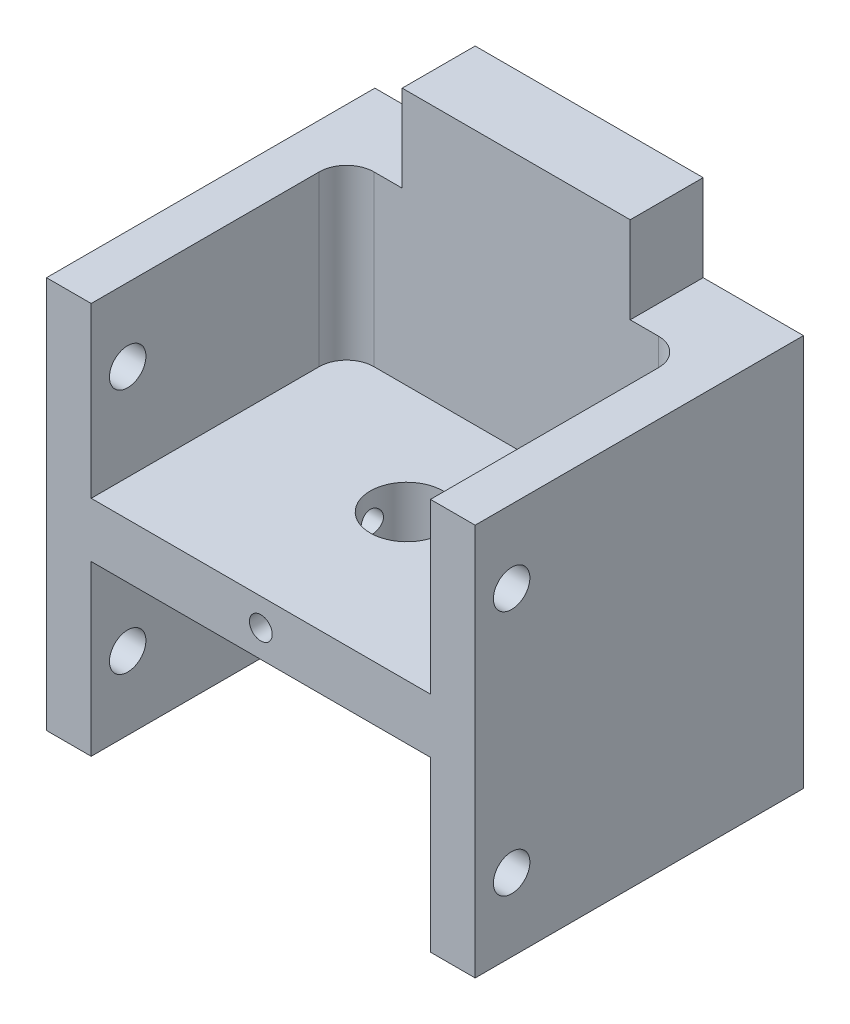
SolidWorks part; units mm, degrees
ref_plane "前视基准面" through (0, 0, 0) normal (0, 0, 1) x (1, 0, 0)
ref_plane "上视基准面" through (0, 0, 0) normal (0, 1, 0) x (1, 0, 0)
ref_plane "右视基准面" through (0, 0, 0) normal (1, 0, 0) x (0, 0, -1)
sketch "草图1" plane through (0, 0, 0) normal (0, 0, 1) x (1, 0, 0)
  line L1 (-23.5, -21.5) -> (23.5, -21.5)
  line L2 (-23.5, -21.5) -> (-23.5, 21.5)
  line L3 (-23.5, 21.5) -> (23.5, 21.5)
  line L4 (23.5, -21.5) -> (23.5, 21.5)
  line L5 (-23.5, -21.5) -> (23.5, 21.5) construction
  line L6 (-23.5, 21.5) -> (23.5, -21.5) construction
  point P0 (0, 0)
  dimension "D1" = 43
  dimension "D2" = 47
extrude "凸台-拉伸1" add sketch "草图1" along normal blind 36
sketch "草图2" plane through (0, 0, 36) normal (0, 0, 1) x (1, 0, 0)
  line L0 (23.5, 21.5) -> (-23.5, 21.5) construction
  line L1 (-18.6, -21.5) -> (18.6, -21.5)
  line L2 (-18.6, -21.5) -> (-18.6, 21.5)
  line L3 (-18.6, 21.5) -> (18.6, 21.5)
  line L4 (18.6, -21.5) -> (18.6, 21.5)
  line L5 (-18.6, -21.5) -> (18.6, 21.5) construction
  line L6 (-18.6, 21.5) -> (18.6, -21.5) construction
  point P0 (0, 0)
  dimension "D1" = 37.2
extrude "切除-拉伸1" cut sketch "草图2" against normal blind 28
sketch "草图3" plane through (-23.5, 0, 0) normal (-1, 0, 0) x (0, 0, 1)
  line L0 (0, 0) -> (36, 0) construction
  line L1 (0, 21.5) -> (0, -21.5) construction
  line L2 (36, 21.5) -> (36, -21.5) construction
  line L3 (36, 21.5) -> (0, 21.5) construction
  circle A0 centre (32, 13.5) radius 2
  circle A2 centre (32, -13.5) radius 2
  dimension "D1" = 4
  dimension "D3" = 4
  dimension "D2" = 8
extrude "切除-拉伸2" cut sketch "草图3" against normal up to surface (47 mm away) up to face at (23.5, 0, 18)
sketch "草图4" plane through (0, 0, 8) normal (0, 0, 1) x (1, 0, 0)
  line L0 (18.6, -21.5) -> (18.6, 21.5) construction
  line L1 (-18.6, -3) -> (18.6, -3)
  line L2 (-18.6, -3) -> (-18.6, 3)
  line L3 (-18.6, 3) -> (18.6, 3)
  line L4 (18.6, -3) -> (18.6, 3)
  line L5 (-18.6, -3) -> (18.6, 3) construction
  line L6 (-18.6, 3) -> (18.6, -3) construction
  point P0 (0, 0)
  dimension "D1" = 6
extrude "凸台-拉伸2" add sketch "草图4" along normal up to surface (28 mm away) up to face at (21.05, 0, 36)
fillet "圆角1" radius 3 4 edges at (18.6, -12.25, 8) (-18.6, -12.25, 8) (-18.6, 12.25, 8) (18.6, 12.25, 8)
sketch "草图5" plane through (0, 3, 0) normal (0, 1, 0) x (1, 0, 0)
  line L0 (-18.6, -36) -> (18.6, -36) construction
  circle A0 centre (0, -20) radius 4
  dimension "D1" = 8
  dimension "D2" = 16
extrude "切除-拉伸3" cut sketch "草图5" against normal up to next
hole_wizard "M3 螺纹孔1" positions "3D草图1" profile "草图6" tap size "M3" standard "GB"
sketch3d "3D草图1"
  line L4 (0, 3, 36) -> (0, -3, 36)
  line L5 (-18.6, 3, 36) -> (18.6, 3, 36) construction
  line L6 (18.6, -3, 36) -> (-18.6, -3, 36) construction
  point P0 (0, 0, 36)
sketch "草图6" plane through (0, 0, 36) normal (1, 0, 0) x (0, -1, 0)
  line L0 (0, 0) -> (0, 12)
  line L1 (0, 12) -> (1.25, 12)
  line L2 (1.25, 12) -> (1.25, 0)
  line L5 (1.25, 0) -> (0, 0)
  line L11 (0, -6.35) -> (0, 107.95) construction
  dimension "通孔螺纹孔钻头直径" = 2.5
  dimension "通孔螺纹孔钻头深度" = 12
cosmetic thread "孔螺蚊线1" parameters "D2"=3
hole_wizard "M3 螺纹孔2" positions "3D草图2" profile "草图7" tap size "M3" standard "GB"
sketch3d "3D草图2"
  line L0 (-23.5, 21.5, 36) -> (-23.5, -21.5, 36) construction
  line L1 (-23.5, 0, 36) -> (-23.5, 0, 20)
  point P0 (-23.5, 0, 20)
  dimension "D1" = 16
sketch "草图7" plane through (-23.5, 0, 20) normal (0, 1, 0) x (0, 0, 1)
  line L0 (0, 0) -> (0, 19.5)
  line L1 (0, 19.5) -> (1.25, 19.5)
  line L2 (1.25, 19.5) -> (1.25, 0)
  line L5 (1.25, 0) -> (0, 0)
  line L11 (0, -6.35) -> (0, 107.95) construction
  dimension "通孔螺纹孔钻头直径" = 2.5
  dimension "通孔螺纹孔钻头深度" = 19.5
cosmetic thread "孔螺蚊线2" parameters "D2"=3
sketch "草图8" plane through (0, 0, 0) normal (0, 0, -1) x (-1, 0, 0)
  line L0 (-23.5, 21.5) -> (23.5, 21.5) construction
  line L1 (-12.5, 31) -> (12.5, 31)
  line L2 (-12.5, 31) -> (-12.5, 21.5)
  line L3 (-12.5, 21.5) -> (12.5, 21.5)
  line L4 (12.5, 31) -> (12.5, 21.5)
  line L5 (-12.5, 31) -> (12.5, 21.5) construction
  line L6 (-12.5, 21.5) -> (12.5, 31) construction
  line L7 (23.5, -21.5) -> (-23.5, -21.5) construction
  line L8 (-12.5, -31) -> (12.5, -31)
  line L9 (-12.5, -31) -> (-12.5, -21.5)
  line L10 (-12.5, -21.5) -> (12.5, -21.5)
  line L11 (12.5, -31) -> (12.5, -21.5)
  line L12 (-12.5, -31) -> (12.5, -21.5) construction
  line L13 (-12.5, -21.5) -> (12.5, -31) construction
  point P0 (0, 26.25)
  point P7 (0, -26.25)
  dimension "D1" = 62
  dimension "D2" = 25
extrude "凸台-拉伸3" add sketch "草图8" against normal up to surface (8 mm away) up to face at (0, 12.25, 8)
sketch "草图9" plane through (-23.5, 0, 0) normal (-1, 0, 0) x (0, 0, 1)
  circle A0 centre (20, 0) radius 2.5
  dimension "D1" = 5
extrude "切除-拉伸4" cut sketch "草图9" against normal blind 14
